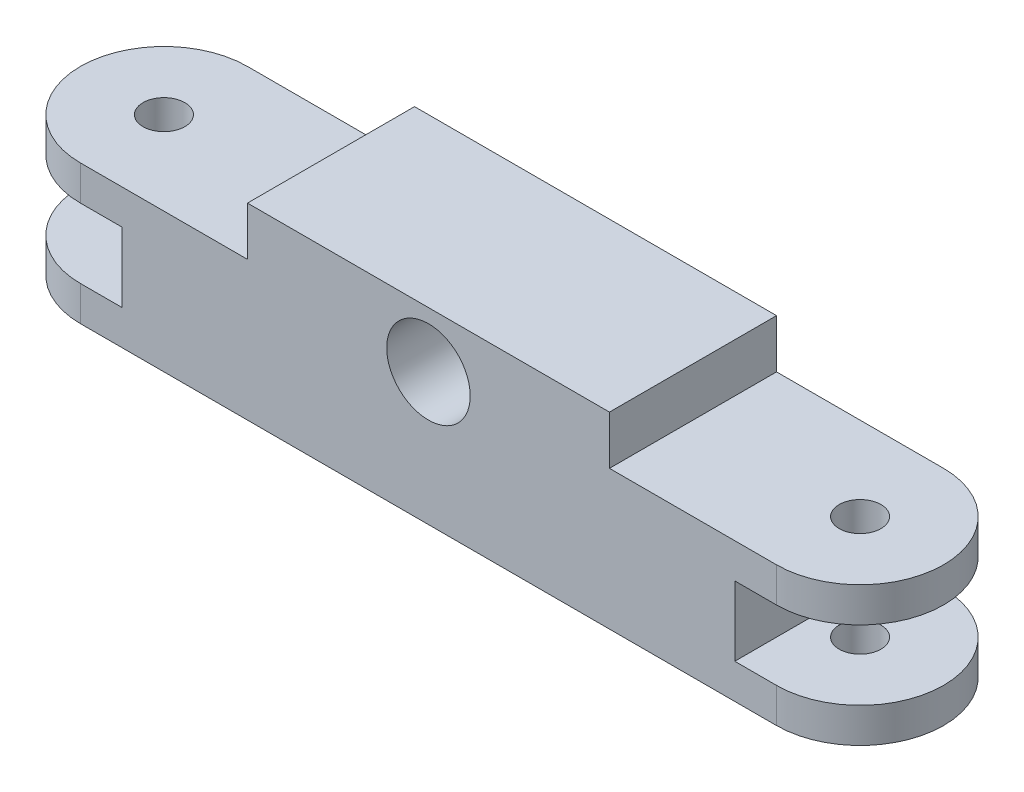
from build123d import *

# Parameters (mm, degrees)
SKETCH1_R           = 1.5
BOSS_EXTRUDE1_DEPTH = 10
SKETCH2_W           = 9
SKETCH2_H           = 5
CUT_EXTRUDE1_DEPTH  = 24.832750576
SKETCH3_W           = 12
SKETCH3_H           = 5
BOSS_EXTRUDE2_DEPTH = 32
SKETCH5_W           = 26
SKETCH5_H           = 6
SKETCH5_H_2         = 2.5
BOSS_EXTRUDE6_DEPTH = 12
SKETCH6_R           = 3
CUT_EXTRUDE2_DEPTH  = 59.840887145


with BuildPart() as part:
    # Sketch1 → Boss-Extrude1 (new body)
    with BuildSketch(Plane(origin=(0, 0, 0), x_dir=(1, 0, 0), z_dir=(0, 1, 0))):
        with BuildLine():
            Line((0, 6), (12, 6))
            ThreePointArc((12, 6), (18, 0), (12, -6))
            Line((12, -6), (0, -6))
            ThreePointArc((0, -6), (-6, 0), (0, 6))
        make_face()
        with Locations(Location((0, 0, 0), (0, 0, 270))):
            Circle(SKETCH1_R, mode=Mode.SUBTRACT)
    extrude(amount=BOSS_EXTRUDE1_DEPTH)

    # Sketch2 → Cut-Extrude1 (cut, through all)
    with BuildSketch(Plane.XY.offset(6)):
        with Locations((-1.5, 5)):
            Rectangle(SKETCH2_W, SKETCH2_H)
        with Locations((13.5, 5)):
            Rectangle(SKETCH2_W, SKETCH2_H)
    extrude(amount=-CUT_EXTRUDE1_DEPTH, mode=Mode.SUBTRACT)

    # Sketch3 → Boss-Extrude2 (add)
    with BuildSketch(Plane(origin=(9, 0, 0), x_dir=(0, 0, -1), z_dir=(1, 0, 0))):
        with Locations((0, 5)):
            Rectangle(SKETCH3_W, SKETCH3_H)
    extrude(amount=BOSS_EXTRUDE2_DEPTH)

    # Mirror1: part across plane


with BuildPart() as part_1:
    add(part.part)
    add(part.part.mirror(Plane(origin=(25, 0, 0), x_dir=(0, 0, 1), z_dir=(1, 0, 0))))

    # Sketch5 → Boss-Extrude6 (add)
    with BuildSketch(Plane.XY.offset(6)):
        with Locations((25, 10.5)):
            Rectangle(SKETCH5_W, SKETCH5_H)
        with Locations((25, 1.25)):
            Rectangle(SKETCH5_W, SKETCH5_H_2)
    extrude(amount=-BOSS_EXTRUDE6_DEPTH)

    # Sketch6 → Cut-Extrude2 (cut, through all)
    with BuildSketch(Plane.XY.offset(6)):
        with Locations((25, 9.5)):
            Circle(SKETCH6_R)
    extrude(amount=-CUT_EXTRUDE2_DEPTH, mode=Mode.SUBTRACT)


solid = part_1.part
